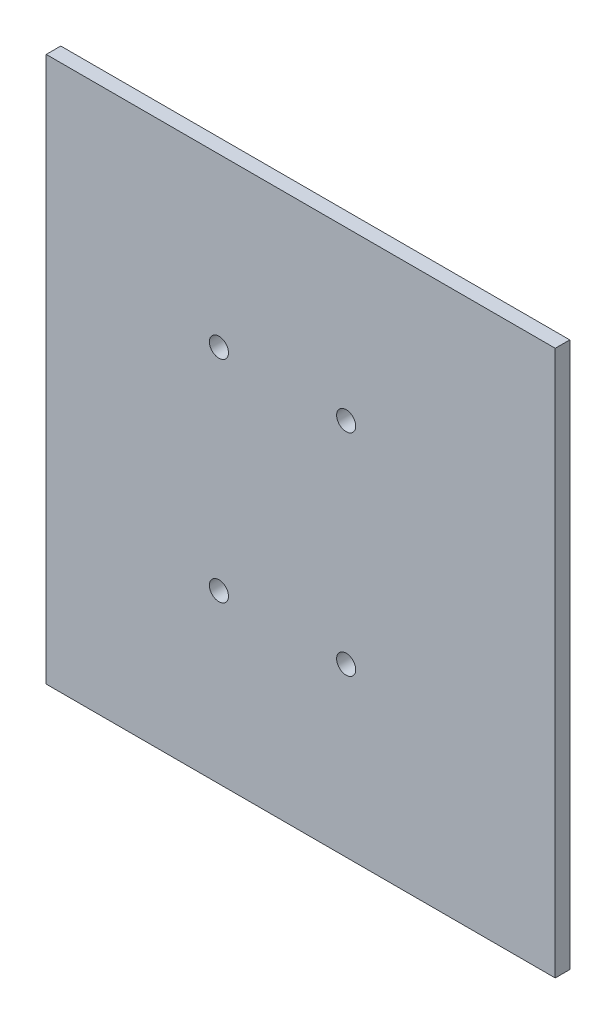
from build123d import *

# Parameters (mm, degrees)
SKETCH1_W           = 280
SKETCH1_H           = 300
BOSS_EXTRUDE1_DEPTH = 8
SKETCH2_R           = 5.25
CUT_EXTRUDE1_DEPTH  = 326.70694063


with BuildPart() as part:
    # Sketch1 → Boss-Extrude1 (new body)
    with BuildSketch(Plane.XY):
        with Locations((58.397782613, -108.184683955)):
            Rectangle(SKETCH1_W, SKETCH1_H)
    extrude(amount=BOSS_EXTRUDE1_DEPTH)

    # Sketch2 → Cut-Extrude1 (cut, through all)
    with BuildSketch(Plane(origin=(0, 0, 0), x_dir=(-1, 0, 0), z_dir=(0, 0, -1))):
        with Locations((-13.397782613, -50.184683955)):
            Circle(SKETCH2_R)
        with Locations((-83.397782613, -50.184683955)):
            Circle(SKETCH2_R)
        with Locations(Location((-13.397782613, -166.184683955, 0), (0, 0, 180))):
            Circle(SKETCH2_R)
        with Locations(Location((-83.397782613, -166.184683955, 0), (0, 0, 180))):
            Circle(SKETCH2_R)
    extrude(amount=-CUT_EXTRUDE1_DEPTH, mode=Mode.SUBTRACT)


solid = part.part
